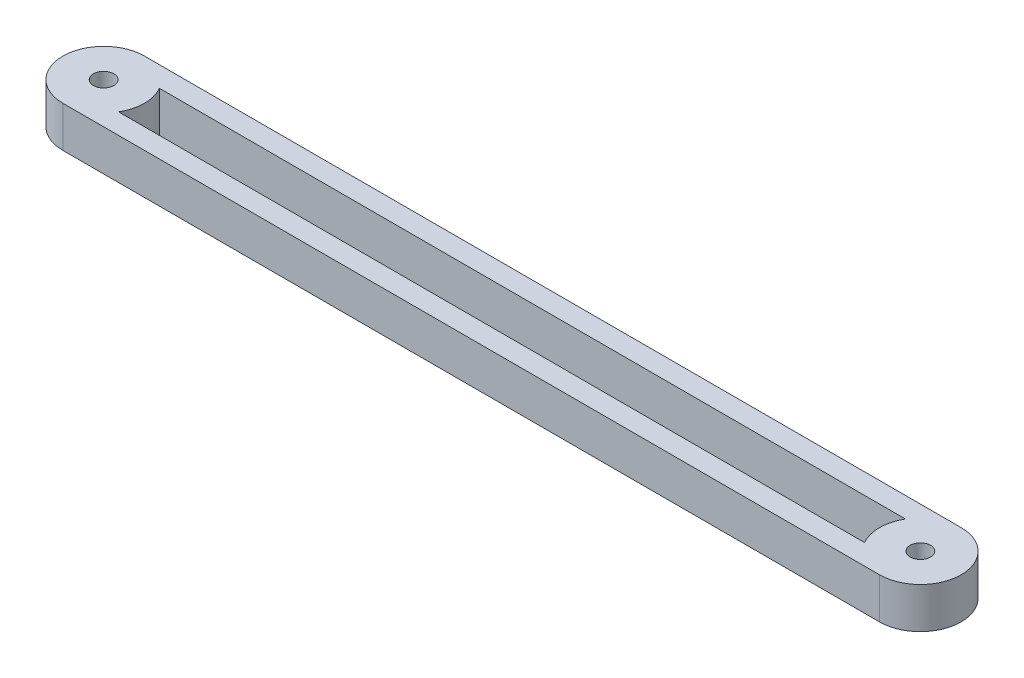
SolidWorks part; units mm, degrees
ref_plane "Front Plane" through (0, 0, 0) normal (0, 0, 1) x (1, 0, 0)
ref_plane "Top Plane" through (0, 0, 0) normal (0, 1, 0) x (1, 0, 0)
ref_plane "Right Plane" through (0, 0, 0) normal (1, 0, 0) x (0, 0, -1)
other "Configuration Table"
sketch "Sketch1" plane through (0, 0, 0) normal (0, 1, 0) x (1, 0, 0)
  line L1 (-200, 20) -> (200, 20)
  line L2 (-200, 20) -> (-200, -20)
  line L3 (-200, -20) -> (200, -20)
  line L4 (200, 20) -> (200, -20)
  line L5 (0, -20) -> (0, 20) construction
  line L6 (-200, 0) -> (200, 0) construction
  point P0 (0, 0)
  dimension "D1" = 400
  dimension "D2" = 40
extrude "Boss-Extrude1" add sketch "Sketch1" along normal blind 20
sketch "Sketch2" plane through (0, 20, 0) normal (0, 1, 0) x (1, 0, 0)
  line L8 (190, -10) -> (190, 10)
  line L9 (190, 10) -> (-190, 10)
  line L10 (-190, 10) -> (-190, -10)
  line L11 (-190, -10) -> (190, -10)
  line L12 (190, -10) -> (190, 10)
  line L13 (190, 10) -> (-190, 10)
  line L14 (-190, 10) -> (-190, -10)
  line L15 (-190, -10) -> (190, -10)
  dimension "D1" = 10
extrude "Cut-Extrude1" cut sketch "Sketch2" against normal through all
sketch "Sketch4" plane through (0, 20, 0) normal (0, 1, 0) x (1, 0, 0)
  line L0 (200, -20) -> (200, 20) construction
  line L1 (0, -11) -> (0, 11) construction
  circle A0 centre (200, 0) radius 20
  circle A1 centre (-200, 0) radius 20
extrude "Boss-Extrude2" add sketch "Sketch4" against normal blind 20
sketch "Sketch6" plane through (0, 20, 0) normal (0, 1, 0) x (1, 0, 0)
  line L0 (0, -11) -> (0, 11) construction
  circle A0 centre (200, 0) radius 5
  circle A1 centre (-200, 0) radius 5
  dimension "D1" = 10
extrude "Cut-Extrude2" cut sketch "Sketch6" against normal through all
